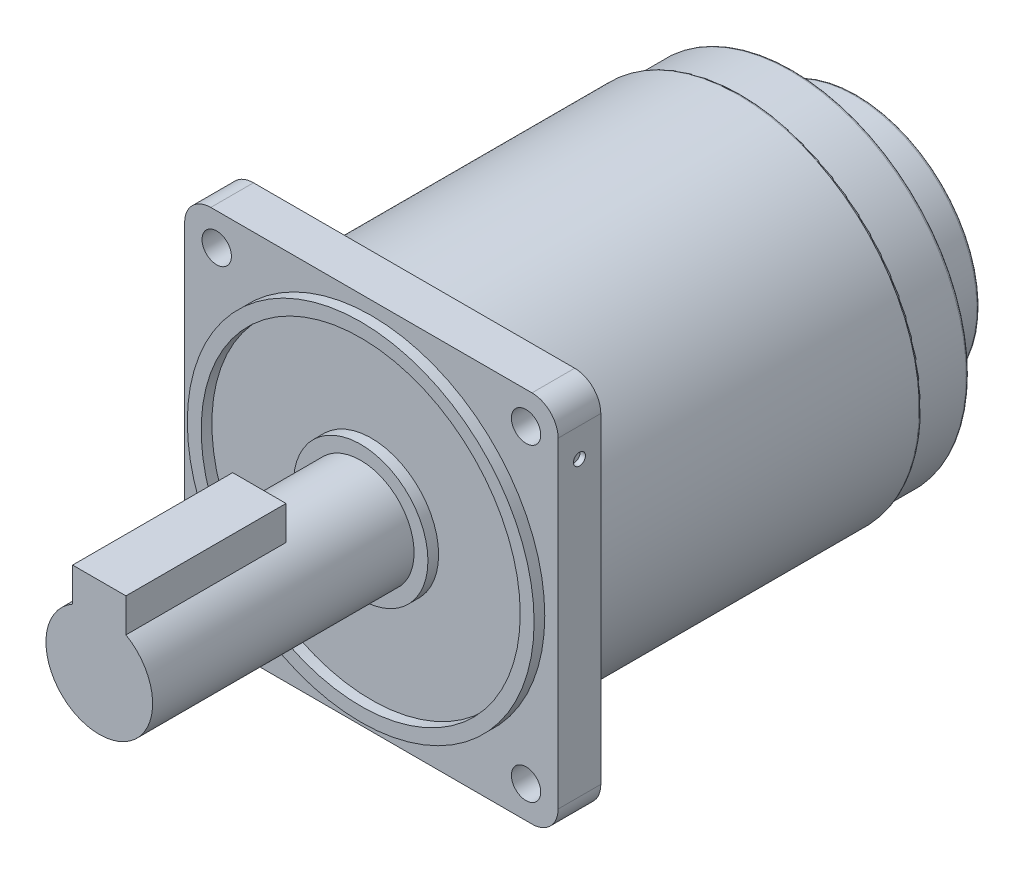
from build123d import *

# Parameters (mm, degrees)
SKETCH_3_W                  = 70
SKETCH_3_H                  = 70
EXTRUDE_1_DEPTH             = 8
SKETCH_5_W                  = 32
SKETCH_5_H                  = 4
SKETCH_5_W_2                = 2
SKETCH_5_H_2                = 2.6
SKETCH_4_R                  = 2.75
CUT_EXTRUDE_1_DEPTH         = 8
PATTERN_CIRCULAR_1_COUNT    = 4
FILLET_1_R                  = 4.9
SKETCH_7_R                  = 1.12
CUT_EXTRUDE_2_DEPTH         = 1
CUT_EXTRUDE_START           = -25
CUT_EXTRUDE_7_DEPTH         = 25
CHAMFER_2_SIZE              = 0.38
SKETCH_35_R                 = 6
EXTRUDE_7_DEPTH             = 4
FILLET_4_R                  = 0.5
SCALE_1_SCALE               = 0.5
EXTRUDE_8_REACH             = 68.293
SKETCH_37_R                 = 5
EXTRUDE_8_DIRECTION_2_DEPTH = 9.5
SKETCH_38_W                 = 5
SKETCH_38_H                 = 5
EXTRUDE_9_DEPTH             = 15


with BuildPart() as part:
    # 草图3 → 凸台-拉伸1 (new body)
    with BuildSketch(Plane.XY):
        Rectangle(SKETCH_3_W, SKETCH_3_H)
    extrude(amount=-EXTRUDE_1_DEPTH)

    # 草图5 → 旋转1 (revolve)
    with BuildSketch(Plane(origin=(0, 0, 0), x_dir=(0, 0, -1), z_dir=(1, 0, 0)), mode=Mode.PRIVATE) as revolve_1_sk:
        with Locations((-16, 2)):
            Rectangle(SKETCH_5_W, SKETCH_5_H)
        with Locations((-1, 31.2)):
            Rectangle(SKETCH_5_W_2, SKETCH_5_H_2)
        with Locations((-1, 11.3)):
            Rectangle(SKETCH_5_W_2, SKETCH_5_H_2)
    revolve(revolve_1_sk.sketch.rotate(Axis((0, 0, 32), (0, 0, -1)), 90), axis=Axis((0, 0, 32), (0, 0, -1)))

    # 草图4 → 切除-拉伸1 (cut)
    with BuildSketch(Plane.XY):
        with Locations((28.991378029, 28.991378029)):
            Circle(SKETCH_4_R)
    cut_extrude_1 = extrude(amount=-CUT_EXTRUDE_1_DEPTH, mode=Mode.SUBTRACT)

    # 阵列(圆周)1: 切除-拉伸1 ×4 about axis
    pattern_circular_1_axis = Axis((0, 0, 0), (0, 0, 1))
    for i in range(1, PATTERN_CIRCULAR_1_COUNT):
        add(cut_extrude_1.rotate(pattern_circular_1_axis, i * 360 / PATTERN_CIRCULAR_1_COUNT), mode=Mode.SUBTRACT)

    # 圆角1
    fillet_1_edges = [part.edges().sort_by_distance(p)[0] for p in [
        (-35, 35, -4),
        (35, 35, -4),
        (35, -35, -4),
        (-35, -35, -4),
    ]]
    fillet(fillet_1_edges, radius=FILLET_1_R)

    # 草图7 → 切除-拉伸2 (cut)
    with BuildSketch(Plane(origin=(35, 0, 0), x_dir=(0, 0, -1), z_dir=(1, 0, 0))):
        with Locations((4, 24.7)):
            Circle(SKETCH_7_R)
    extrude(amount=-CUT_EXTRUDE_2_DEPTH, mode=Mode.SUBTRACT)

    # 草图31 → 切除-拉伸7 (cut)
    with BuildSketch(Plane.XY.offset(32).offset(CUT_EXTRUDE_START)):
        with BuildLine():
            Line((3.5, 1.936491673), (3.5, -1.936491673))
            ThreePointArc((3.5, -1.936491673), (4, 0), (3.5, 1.936491673))
        make_face()
    extrude(amount=CUT_EXTRUDE_7_DEPTH, mode=Mode.SUBTRACT)

    # 倒角2
    chamfer_2_edges = [part.edges().sort_by_distance(p)[0] for p in [
        (-4, 0, 32),
    ]]
    chamfer(chamfer_2_edges, length=CHAMFER_2_SIZE)

    # 草图35 → 凸台-拉伸7 (add)
    with BuildSketch(Plane.XY):
        Circle(SKETCH_35_R)
    extrude(amount=EXTRUDE_7_DEPTH)

    # 草图8 → 旋转3 (revolve)
    with BuildSketch(Plane(origin=(0, 0, 0), x_dir=(0, 0, -1), z_dir=(1, 0, 0))):
        Polygon((8, 34), (69.2, 34), (69.2, 33), (79, 33), (79, 23), (91, 23), (91, 0), (8, 0), align=None)
    revolve(axis=Axis((0, 0, -91), (0, 0, 1)))

    # 圆角4
    fillet_4_edges = [part.edges().sort_by_distance(p)[0] for p in [
        (0, -34, -69.2),
        (0, -33, -79),
        (0, -23, -91),
    ]]
    fillet(fillet_4_edges, radius=FILLET_4_R)


with BuildPart() as part_1:
    # 缩放比例1: scaled about (-0.000807306, -0.000306882, -40.615231306)
    add(part.part.scale(SCALE_1_SCALE).moved(Location((-0.000403653, -0.000153441, -20.307615653))))

    # 草图37 → 凸台-拉伸8 (add, up to next)
    with BuildSketch(Plane.XY.offset(-4.307615654), mode=Mode.PRIVATE) as extrude_8_sk1:
        with Locations(Location((0, 0, 0), (0, 0, 110.815805109))):
            Circle(SKETCH_37_R)
    extrude_8_tool1 = extrude(extrude_8_sk1.sketch, amount=-EXTRUDE_8_REACH, mode=Mode.PRIVATE) - part_1.part
    add(extrude_8_tool1.solids().sort_by_distance((0, 0, -4.307616))[0])

    # 草图37 → 凸台-拉伸8 direction 2 (add)
    with BuildSketch(Plane.XY.offset(-4.307615654)):
        with Locations(Location((0, 0, 0), (0, 0, 110.815805109))):
            Circle(SKETCH_37_R)
    extrude(amount=EXTRUDE_8_DIRECTION_2_DEPTH)

    # 草图38 → 凸台-拉伸9 (add)
    with BuildSketch(Plane.XY.offset(5.192384346)):
        with Locations((0, 5)):
            Rectangle(SKETCH_38_W, SKETCH_38_H)
    extrude(amount=-EXTRUDE_9_DEPTH)


solid = part_1.part
